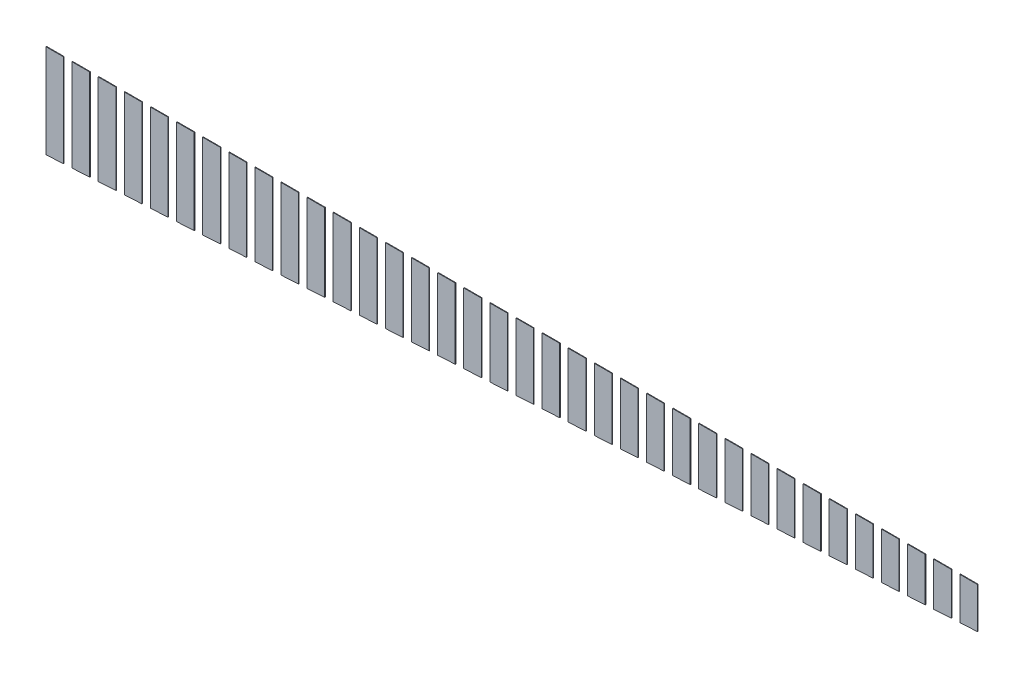
SolidWorks part; units mm, degrees
material "AISI 316 stainless steel plate (SS)"
ref_plane "Front Plane" through (0, 0, 0) normal (0, 0, 1) x (1, 0, 0)
ref_plane "Top Plane" through (0, 0, 0) normal (0, 1, 0) x (1, 0, 0)
ref_plane "Right Plane" through (0, 0, 0) normal (1, 0, 0) x (0, 0, -1)
other "Configuration Table"
sketch "Sketch1" plane through (0, 0, 0) normal (0, 0, 1) x (1, 0, 0)
  line L1 (-89.25, -9.5) -> (89.25, -9.5)
  line L2 (-89.25, -9.5) -> (-89.25, 9.5)
  line L3 (-89.25, 9.5) -> (89.25, 9.5)
  line L4 (89.25, -9.5) -> (89.25, 9.5)
  line L5 (-89.25, -9.5) -> (89.25, 9.5) construction
  line L6 (-89.25, 9.5) -> (89.25, -9.5) construction
  point P0 (0, 0)
  dimension "D1" = 19
  dimension "D2" = 178.5
extrude "Boss-Extrude1" add sketch "Sketch1" along normal blind 0.1
sketch "Sketch2" plane through (0, 0, 0.1) normal (0, 0, 1) x (1, 0, 0)
  line L0 (-77.71, 7.7) -> (-74.81, 7.7)
  line L5 (-104.7623, 25.4127) -> (109.6999, 25.4127)
  line L6 (-104.7623, 25.4127) -> (-104.7623, -33.1406)
  line L349 (-104.7623, -33.1406) -> (109.6999, -33.1406)
  line L350 (109.6999, 25.4127) -> (109.6999, -33.1406)
  line L351 (-74.81, 7.7) -> (-74.81, -7.5475)
  line L352 (-77.71, -7.7116) -> (-74.81, -7.5475)
  line L353 (-77.71, 7.7) -> (-77.71, -7.7116)
  line L354 (-73.41, 7.7) -> (-70.51, 7.7)
  line L355 (-70.51, 7.7) -> (-70.51, -7.3041)
  line L356 (-73.41, -7.4682) -> (-70.51, -7.3041)
  line L357 (-73.41, 7.7) -> (-73.41, -7.4682)
  line L358 (-69.11, 7.7) -> (-66.21, 7.7)
  line L359 (-66.21, 7.7) -> (-66.21, -7.0606)
  line L360 (-69.11, -7.2248) -> (-66.21, -7.0606)
  line L361 (-69.11, 7.7) -> (-69.11, -7.2248)
  line L362 (-64.81, 7.7) -> (-61.91, 7.7)
  line L363 (-61.91, 7.7) -> (-61.91, -6.8172)
  line L364 (-64.81, -6.9814) -> (-61.91, -6.8172)
  line L365 (-64.81, 7.7) -> (-64.81, -6.9814)
  line L366 (-60.51, 7.7) -> (-57.61, 7.7)
  line L367 (-57.61, 7.7) -> (-57.61, -6.5738)
  line L368 (-60.51, -6.738) -> (-57.61, -6.5738)
  line L369 (-60.51, 7.7) -> (-60.51, -6.738)
  line L370 (-56.21, 7.7) -> (-53.31, 7.7)
  line L371 (-53.31, 7.7) -> (-53.31, -6.3304)
  line L372 (-56.21, -6.4945) -> (-53.31, -6.3304)
  line L374 (-56.21, 7.7) -> (-56.21, -6.4945)
  line L375 (-51.91, 7.7) -> (-49.01, 7.7)
  line L376 (-49.01, 7.7) -> (-49.01, -6.087)
  line L377 (-51.91, -6.2511) -> (-49.01, -6.087)
  line L386 (-51.91, 7.7) -> (-51.91, -6.2511)
  line L387 (-47.61, 7.7) -> (-44.71, 7.7)
  line L388 (-44.71, 7.7) -> (-44.71, -5.8435)
  line L389 (-47.61, -6.0077) -> (-44.71, -5.8435)
  line L390 (-47.61, 7.7) -> (-47.61, -6.0077)
  line L391 (-43.31, 7.7) -> (-40.41, 7.7)
  line L393 (-40.41, 7.7) -> (-40.41, -5.6001)
  line L431 (-43.31, -5.7643) -> (-40.41, -5.6001)
  line L432 (-43.31, 7.7) -> (-43.31, -5.7643)
  line L433 (-39.01, 7.7) -> (-36.11, 7.7)
  line L434 (-36.11, 7.7) -> (-36.11, -5.3567)
  line L435 (-39.01, -5.5209) -> (-36.11, -5.3567)
  line L436 (-39.01, 7.7) -> (-39.01, -5.5209)
  line L437 (-34.71, 7.7) -> (-31.81, 7.7)
  line L438 (-31.81, 7.7) -> (-31.81, -5.1133)
  line L439 (-34.71, -5.2775) -> (-31.81, -5.1133)
  line L440 (-34.71, 7.7) -> (-34.71, -5.2775)
  line L441 (-30.41, 7.7) -> (-27.51, 7.7)
  line L442 (-27.51, 7.7) -> (-27.51, -4.8699)
  line L443 (-30.41, -5.034) -> (-27.51, -4.8699)
  line L444 (-30.41, 7.7) -> (-30.41, -5.034)
  line L445 (-26.11, 7.7) -> (-23.21, 7.7)
  line L446 (-23.21, 7.7) -> (-23.21, -4.6265)
  line L447 (-26.11, -4.7906) -> (-23.21, -4.6265)
  line L448 (-26.11, 7.7) -> (-26.11, -4.7906)
  line L449 (-21.81, 7.7) -> (-18.91, 7.7)
  line L450 (-18.91, 7.7) -> (-18.91, -4.383)
  line L451 (-21.81, -4.5472) -> (-18.91, -4.383)
  line L452 (-21.81, 7.7) -> (-21.81, -4.5472)
  line L453 (-17.51, 7.7) -> (-14.61, 7.7)
  line L454 (-14.61, 7.7) -> (-14.61, -4.1396)
  line L455 (-17.51, -4.3038) -> (-14.61, -4.1396)
  line L456 (-17.51, 7.7) -> (-17.51, -4.3038)
  line L457 (-13.21, 7.7) -> (-10.31, 7.7)
  line L458 (-10.31, 7.7) -> (-10.31, -3.8962)
  line L459 (-13.21, -4.0604) -> (-10.31, -3.8962)
  line L460 (-13.21, 7.7) -> (-13.21, -4.0604)
  line L461 (-8.91, 7.7) -> (-6.01, 7.7)
  line L462 (-6.01, 7.7) -> (-6.01, -3.6528)
  line L463 (-8.91, -3.8169) -> (-6.01, -3.6528)
  line L464 (-8.91, 7.7) -> (-8.91, -3.8169)
  line L465 (-4.61, 7.7) -> (-1.71, 7.7)
  line L466 (-1.71, 7.7) -> (-1.71, -3.4094)
  line L467 (-4.61, -3.5735) -> (-1.71, -3.4094)
  line L468 (-4.61, 7.7) -> (-4.61, -3.5735)
  line L469 (-0.31, 7.7) -> (2.59, 7.7)
  line L470 (2.59, 7.7) -> (2.59, -3.1659)
  line L471 (-0.31, -3.3301) -> (2.59, -3.1659)
  line L472 (-0.31, 7.7) -> (-0.31, -3.3301)
  line L473 (3.99, 7.7) -> (6.89, 7.7)
  line L474 (6.89, 7.7) -> (6.89, -2.9225)
  line L475 (3.99, -3.0867) -> (6.89, -2.9225)
  line L476 (3.99, 7.7) -> (3.99, -3.0867)
  line L477 (8.29, 7.7) -> (11.19, 7.7)
  line L478 (11.19, 7.7) -> (11.19, -2.6791)
  line L479 (8.29, -2.8433) -> (11.19, -2.6791)
  line L480 (8.29, 7.7) -> (8.29, -2.8433)
  line L481 (12.59, 7.7) -> (15.49, 7.7)
  line L482 (15.49, 7.7) -> (15.49, -2.4357)
  line L483 (12.59, -2.5998) -> (15.49, -2.4357)
  line L484 (12.59, 7.7) -> (12.59, -2.5998)
  line L485 (16.89, 7.7) -> (19.79, 7.7)
  line L486 (19.79, 7.7) -> (19.79, -2.1923)
  line L487 (16.89, -2.3564) -> (19.79, -2.1923)
  line L488 (16.89, 7.7) -> (16.89, -2.3564)
  line L489 (21.19, 7.7) -> (24.09, 7.7)
  line L490 (24.09, 7.7) -> (24.09, -1.9488)
  line L491 (21.19, -2.113) -> (24.09, -1.9488)
  line L492 (21.19, 7.7) -> (21.19, -2.113)
  line L493 (25.49, 7.7) -> (28.39, 7.7)
  line L494 (28.39, 7.7) -> (28.39, -1.7054)
  line L495 (25.49, -1.8696) -> (28.39, -1.7054)
  line L496 (25.49, 7.7) -> (25.49, -1.8696)
  line L497 (29.79, 7.7) -> (32.69, 7.7)
  line L498 (32.69, 7.7) -> (32.69, -1.462)
  line L499 (29.79, -1.6262) -> (32.69, -1.462)
  line L500 (29.79, 7.7) -> (29.79, -1.6262)
  line L501 (34.09, 7.7) -> (36.99, 7.7)
  line L502 (36.99, 7.7) -> (36.99, -1.2186)
  line L503 (34.09, -1.3828) -> (36.99, -1.2186)
  line L504 (34.09, 7.7) -> (34.09, -1.3828)
  line L505 (38.39, 7.7) -> (41.29, 7.7)
  line L506 (41.29, 7.7) -> (41.29, -0.9752)
  line L507 (38.39, -1.1393) -> (41.29, -0.9752)
  line L508 (38.39, 7.7) -> (38.39, -1.1393)
  line L509 (42.69, 7.7) -> (45.59, 7.7)
  line L510 (45.59, 7.7) -> (45.59, -0.7317)
  line L511 (42.69, -0.8959) -> (45.59, -0.7317)
  line L512 (42.69, 7.7) -> (42.69, -0.8959)
  line L513 (46.99, 7.7) -> (49.89, 7.7)
  line L514 (49.89, 7.7) -> (49.89, -0.4883)
  line L515 (46.99, -0.6525) -> (49.89, -0.4883)
  line L516 (46.99, 7.7) -> (46.99, -0.6525)
  line L517 (51.29, 7.7) -> (54.19, 7.7)
  line L518 (54.19, 7.7) -> (54.19, -0.2449)
  line L519 (51.29, -0.4091) -> (54.19, -0.2449)
  line L520 (51.29, 7.7) -> (51.29, -0.4091)
  line L521 (55.59, 7.7) -> (58.49, 7.7)
  line L522 (58.49, 7.7) -> (58.49, -0.0015)
  line L523 (55.59, -0.1657) -> (58.49, -0.0015)
  line L524 (55.59, 7.7) -> (55.59, -0.1657)
  line L525 (59.89, 7.7) -> (62.79, 7.7)
  line L526 (62.79, 7.7) -> (62.79, 0.2419)
  line L527 (59.89, 0.0778) -> (62.79, 0.2419)
  line L528 (59.89, 7.7) -> (59.89, 0.0778)
  line L529 (64.19, 7.7) -> (67.09, 7.7)
  line L530 (67.09, 7.7) -> (67.09, 0.4853)
  line L531 (64.19, 0.3212) -> (67.09, 0.4853)
  line L532 (64.19, 7.7) -> (64.19, 0.3212)
  line L533 (68.49, 7.7) -> (71.39, 7.7)
  line L534 (71.39, 7.7) -> (71.39, 0.7288)
  line L535 (68.49, 0.5646) -> (71.39, 0.7288)
  line L536 (68.49, 7.7) -> (68.49, 0.5646)
  line L537 (72.79, 7.7) -> (75.69, 7.7)
  line L538 (75.69, 7.7) -> (75.69, 0.9722)
  line L539 (72.79, 0.808) -> (75.69, 0.9722)
  line L540 (72.79, 7.7) -> (72.79, 0.808)
extrude "Cut-Extrude1" cut sketch "Sketch2" against normal blind 10
